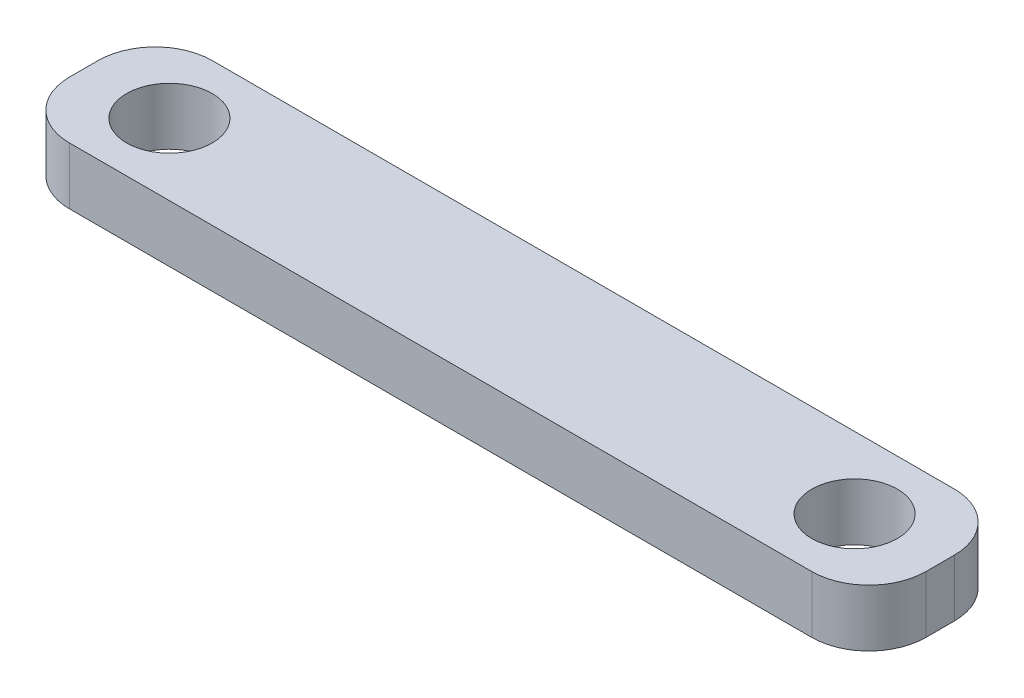
SolidWorks part; units mm, degrees
ref_plane "Front Plane" through (0, 0, 0) normal (0, 0, 1) x (1, 0, 0)
ref_plane "Top Plane" through (0, 0, 0) normal (0, 1, 0) x (1, 0, 0)
ref_plane "Right Plane" through (0, 0, 0) normal (1, 0, 0) x (0, 0, -1)
sketch "Sketch1" plane through (0, 0, 0) normal (0, 1, 0) x (1, 0, 0)
  line L1 (-13, -2.5) -> (13, -2.5)
  line L2 (-15, -0.5) -> (-15, 0.5)
  line L3 (-13, 2.5) -> (13, 2.5)
  line L4 (15, -0.5) -> (15, 0.5)
  line L5 (-15, -2.5) -> (15, 2.5) construction
  line L6 (-15, 2.5) -> (15, -2.5) construction
  line L7 (-15, 0) -> (15, 0) construction
  circle A0 centre (12, 0) radius 1.5
  circle A1 centre (-12, 0) radius 1.5
  arc A2 (15, 0.5) -> (13, 2.5) centre (13, 0.5) ccw
  arc A3 (15, -0.5) -> (13, -2.5) centre (13, -0.5) cw
  arc A4 (-13, -2.5) -> (-15, -0.5) centre (-13, -0.5) cw
  arc A5 (-15, 0.5) -> (-13, 2.5) centre (-13, 0.5) cw
  point P0 (0, 0)
  dimension "D3" = 3
  dimension "D4" = 3
  dimension "D7" = 2
  dimension "D1" = 30
  dimension "D2" = 5
  dimension "D5" = 3
  dimension "D6" = 3
extrude "Boss-Extrude1" add sketch "Sketch1" along normal blind 2
